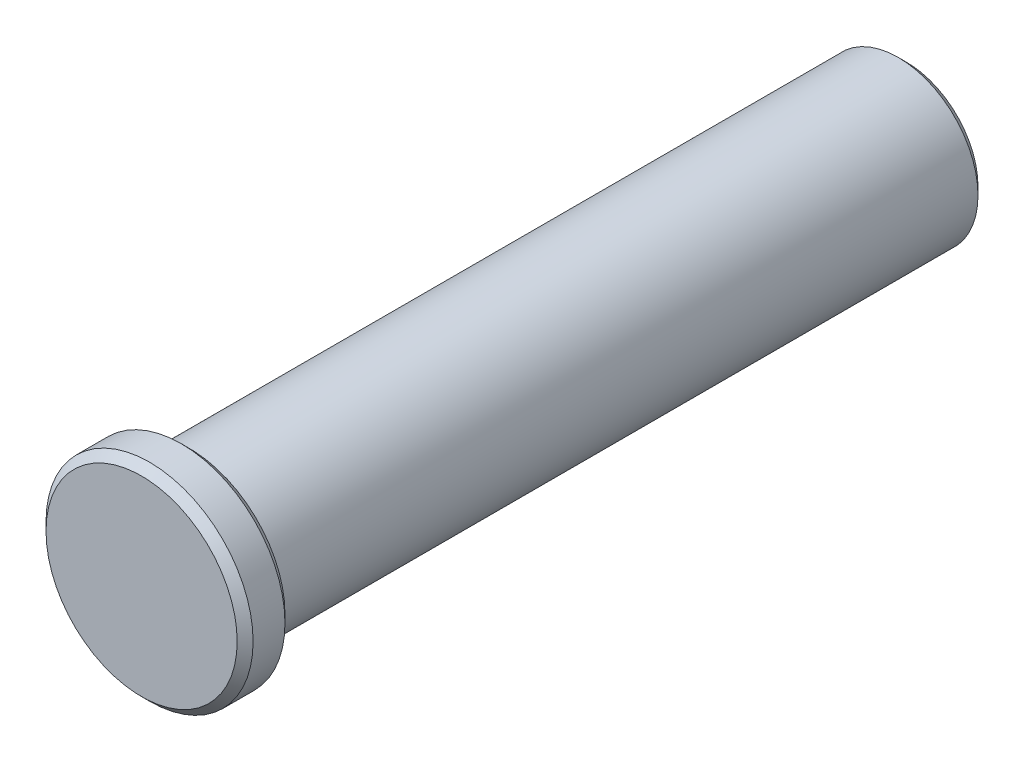
SolidWorks part; units mm, degrees
ref_plane "Front Plane" through (0, 0, 0) normal (0, 0, 1) x (1, 0, 0)
ref_plane "Top Plane" through (0, 0, 0) normal (0, 1, 0) x (1, 0, 0)
ref_plane "Right Plane" through (0, 0, 0) normal (1, 0, 0) x (0, 0, -1)
sketch "Sketch1" plane through (0, 0, 0) normal (0, 0, 1) x (1, 0, 0)
  circle A0 centre (0, 0) radius 5
  dimension "D1" = 10
extrude "Boss-Extrude1" add sketch "Sketch1" along normal blind 45
sketch "Sketch2" plane through (0, 0, 45) normal (0, 0, 1) x (1, 0, 0)
  circle A0 centre (0, 0) radius 6.5
  dimension "D1" = 13
extrude "Boss-Extrude2" add sketch "Sketch2" along normal blind 3
chamfer "Chamfer1" distance 0.5 angle 45 3 edges at (6.5, 0, 48) (6.5, 0, 45) (5, 0, 0)
